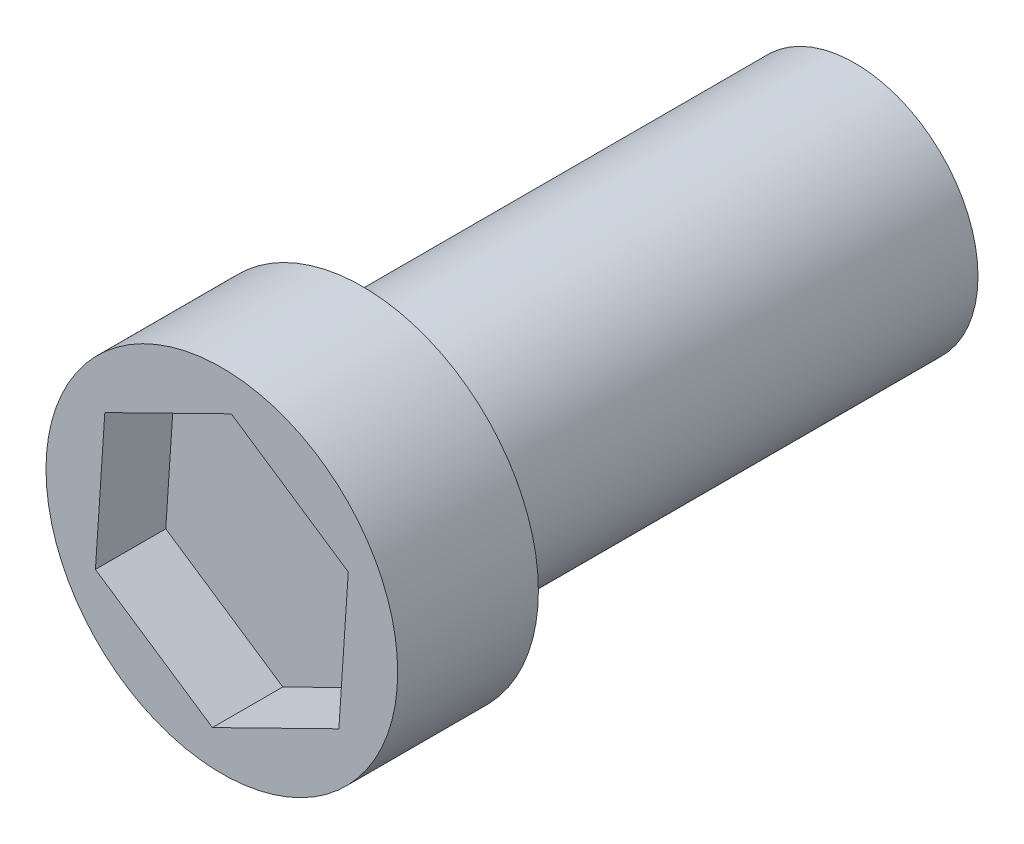
from build123d import *

# Parameters (mm, degrees)
SKETCH1_R           = 2.5
BOSS_EXTRUDE1_DEPTH = 2
CUT_EXTRUDE1_DEPTH  = 1
SKETCH3_R           = 1.75
BOSS_EXTRUDE2_DEPTH = 7


with BuildPart() as part:
    # Sketch1 → Boss-Extrude1 (new body)
    with BuildSketch(Plane.XY):
        Circle(SKETCH1_R)
    extrude(amount=BOSS_EXTRUDE1_DEPTH)

    # Sketch2 → Cut-Extrude1 (cut)
    with BuildSketch(Plane.XY.offset(2)):
        Polygon((1.663695781, -1.114955786), (1.797427926, 0.883324918), (0.133732144, 1.998280704), (-1.663695781, 1.114955786), (-1.797427926, -0.883324918), (-0.133732144, -1.998280704), align=None)
    extrude(amount=-CUT_EXTRUDE1_DEPTH, mode=Mode.SUBTRACT)

    # Sketch3 → Boss-Extrude2 (add)
    with BuildSketch(Plane(origin=(0, 0, 0), x_dir=(-1, 0, 0), z_dir=(0, 0, -1))):
        Circle(SKETCH3_R)
    extrude(amount=BOSS_EXTRUDE2_DEPTH)


solid = part.part
